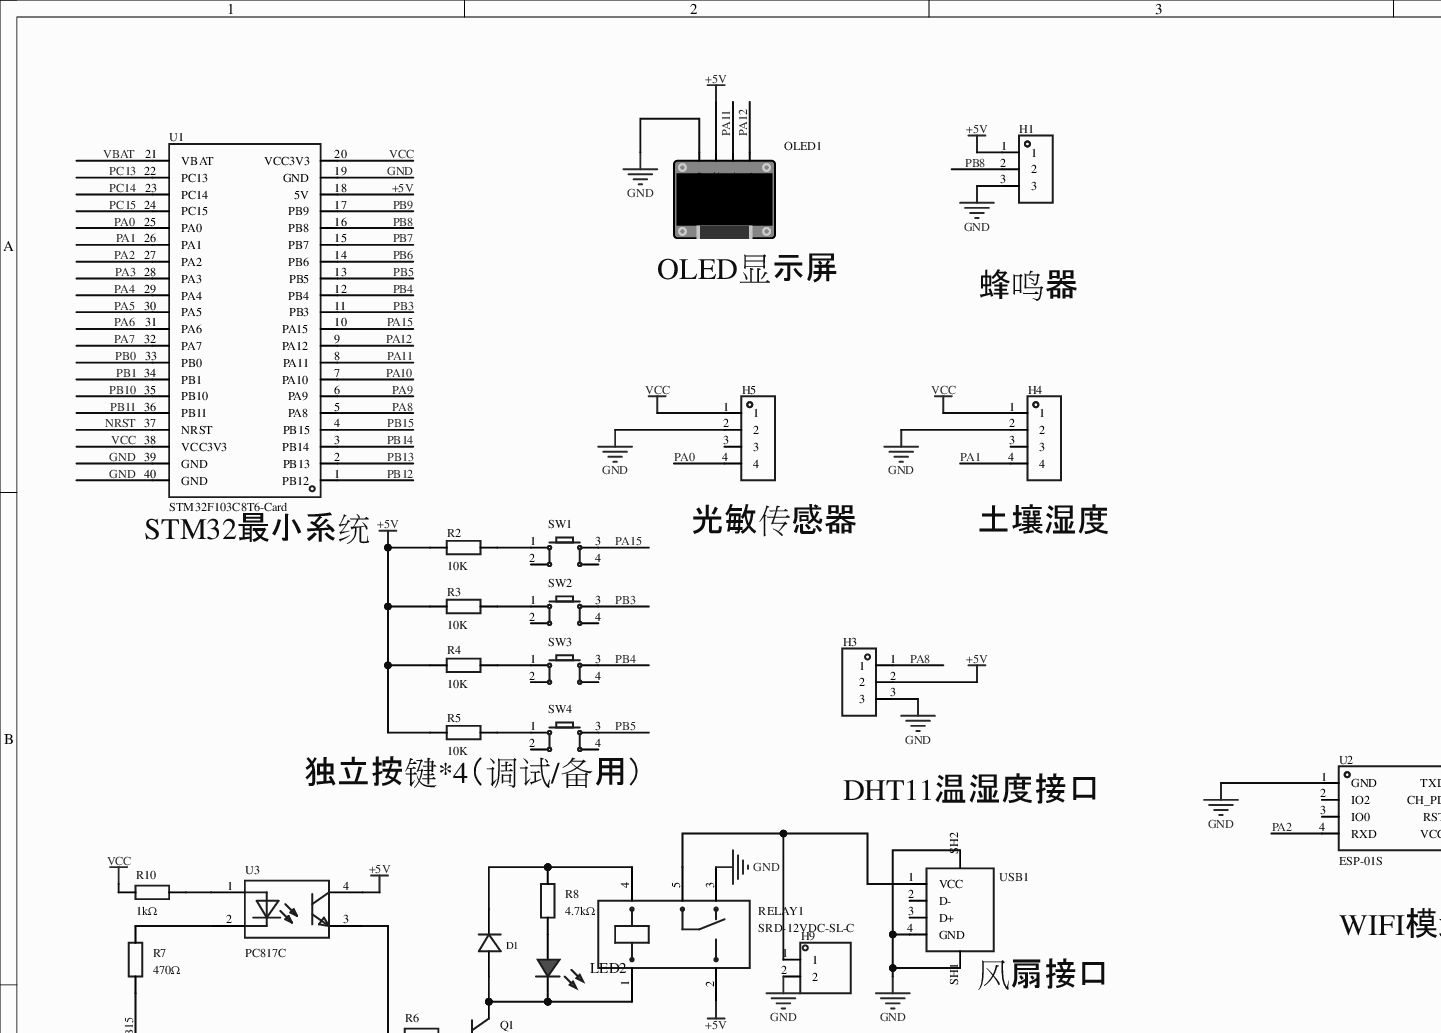
[diagram p0: MISC51241-3.schdoc, top left]
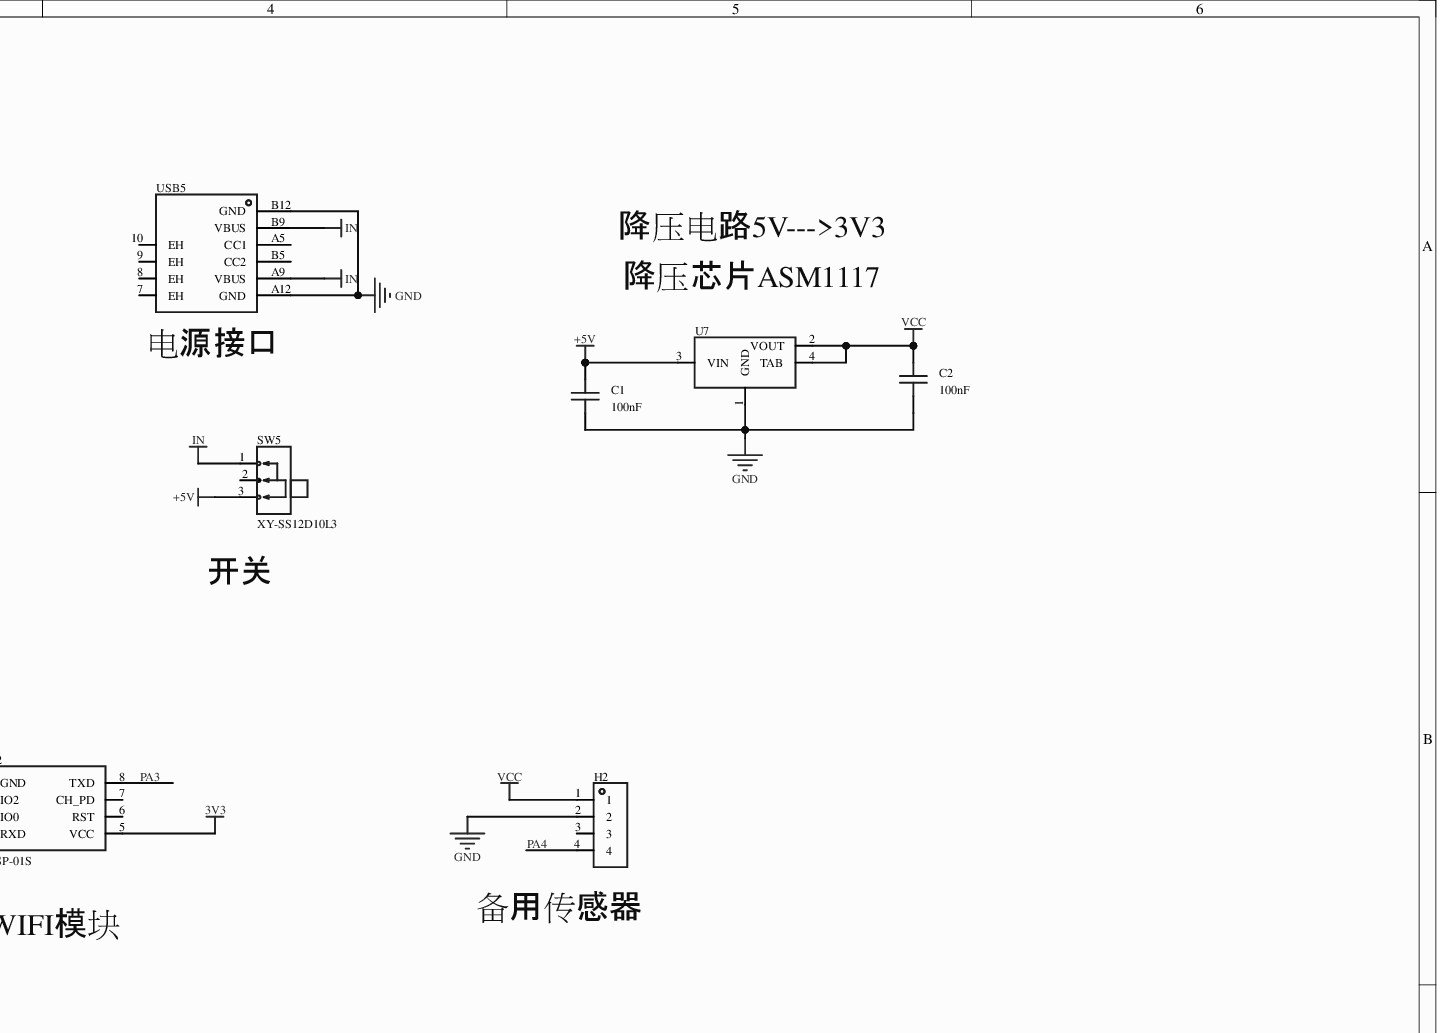
[diagram p1: MISC51241-3.schdoc, top right]
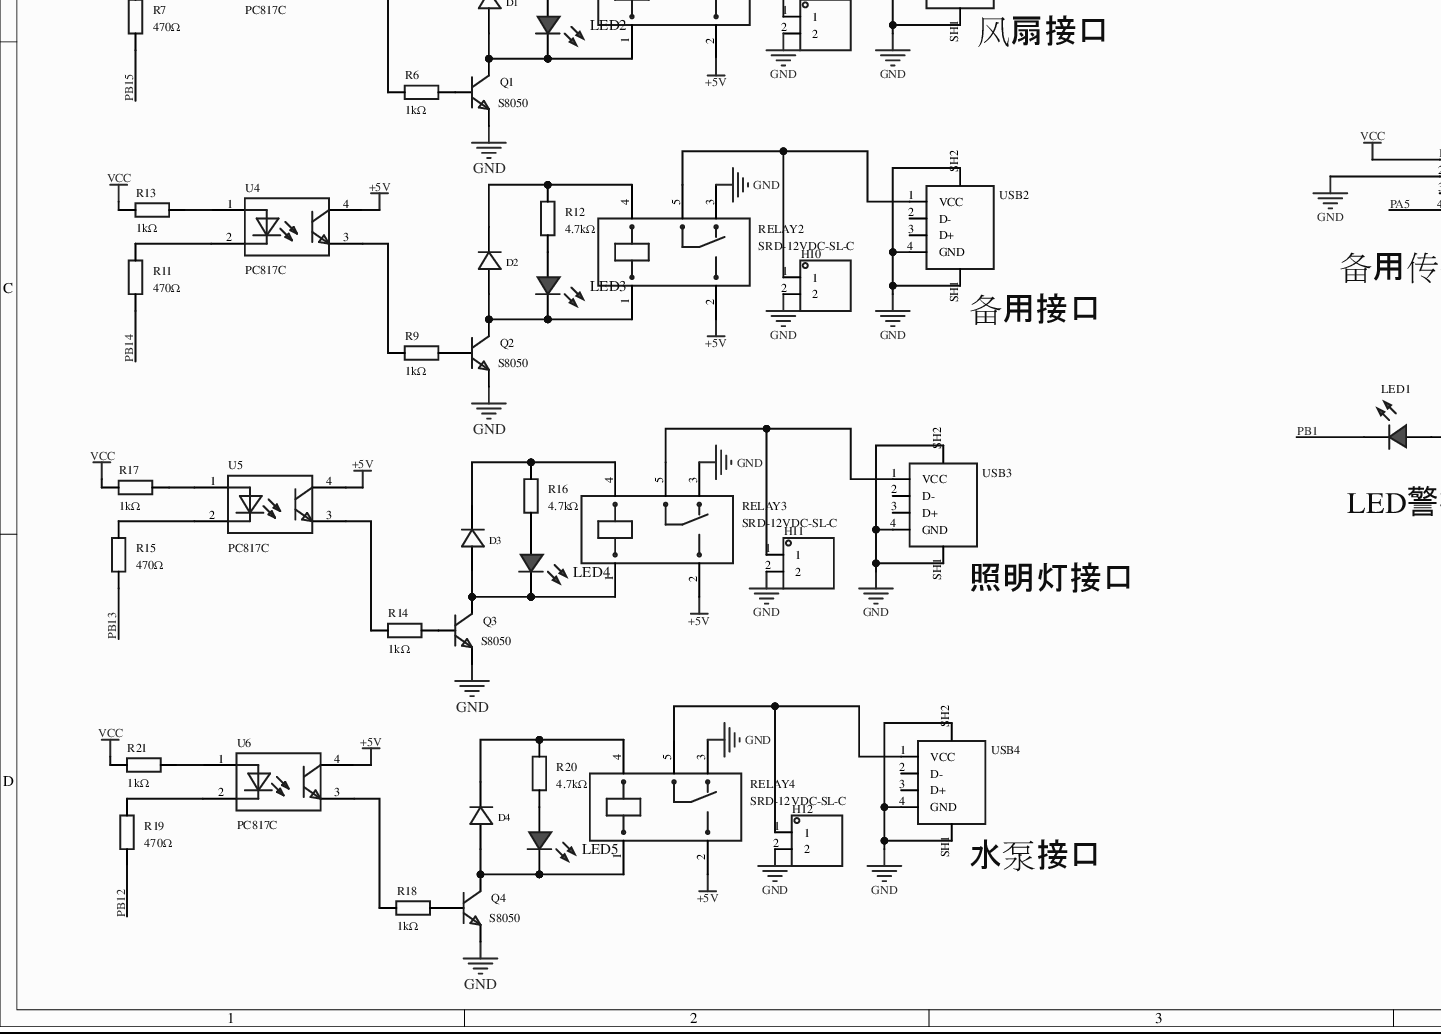
[diagram p2: MISC51241-3.schdoc, bottom left]
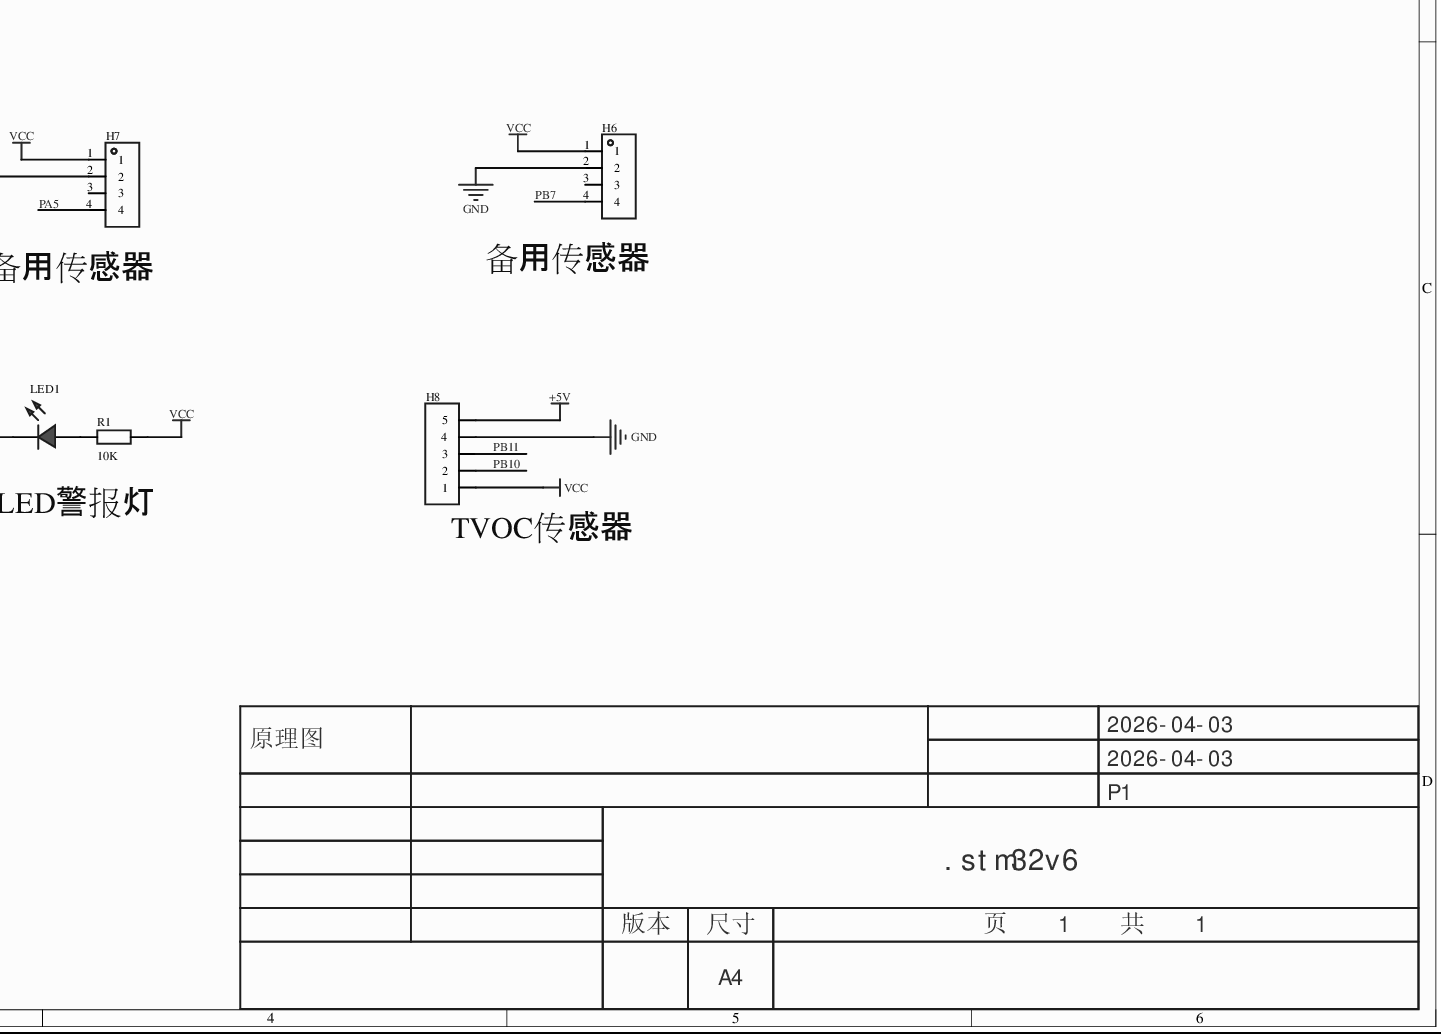
[diagram p3: MISC51241-3.schdoc, bottom right]
# Altium project MISC51241-2.PrjPcb
1 sheet, 70 parts. Net scope: global (net labels, ports and power ports of the same name join across sheets).
Board file: MISC51241.pcbdoc

## Sheet MISC51241-3.schdoc
size 420 x 297 mm; Version: V1.0; @Project Name: MISC51241; @Page Count: 1; @Update Date: 2026-04-03; @Create Date: 2026-04-03; @Schematic Name: MISC51241; @Page No: 1; @Create Time: 23:22:16; @Update Time: 17:32:40; @Board Name: MISC51241

### Parts
C1  100nF  [C0603]
C2  100nF  [C0603]
D1  US1M  [SMA_L4.4-W2.8-LS5.4-RD]  (value not drawn)
D2  US1M  [SMA_L4.4-W2.8-LS5.4-RD]  (value not drawn)
D3  US1M  [SMA_L4.4-W2.8-LS5.4-RD]  (value not drawn)
D4  US1M  [SMA_L4.4-W2.8-LS5.4-RD]  (value not drawn)
H1  (no value)  [HDR-TH_3P-P2.54-V-F]
H2  (no value)  [HDR-TH_4P-P2.54-V-F]
H3  (no value)  [HDR-TH_3P-P2.54-V-F]
H4  (no value)  [HDR-TH_4P-P2.54-V-F]
H5  (no value)  [HDR-TH_4P-P2.54-V-F]
H6  (no value)  [HDR-TH_4P-P2.54-V-F]
H7  (no value)  [HDR-TH_4P-P2.54-V-F]
H8  (no value)  [HDR-TH_5P-P2.54-V-F]
H9  (no value)  [HDR-TH_2P-P2.54-V-M-1]
H10  (no value)  [HDR-TH_2P-P2.54-V-M-1]
H11  (no value)  [HDR-TH_2P-P2.54-V-M-1]
H12  (no value)  [HDR-TH_2P-P2.54-V-M-1]
LED1  (no value)  [LED-TH_5mm]
LED2  (no value)  [LED_0603]
LED3  (no value)  [LED_0603]
LED4  (no value)  [LED_0603]
LED5  (no value)  [LED_0603]
OLED1  (no value)  [0.96OLED_4P]
Q1  S8050  [SOT-23-3_L2.9-W1.6-P1.90-LS2.8-BR]
Q2  S8050  [SOT-23-3_L2.9-W1.6-P1.90-LS2.8-BR]
Q3  S8050  [SOT-23-3_L2.9-W1.6-P1.90-LS2.8-BR]
Q4  S8050  [SOT-23-3_L2.9-W1.6-P1.90-LS2.8-BR]
R1  10K  [R0603]
R2  10K  [R0603]
R3  10K  [R0603]
R4  10K  [R0603]
R5  10K  [R0603]
R6  1kΩ  [R0603]
R7  470Ω  [R0603]
R8  4.7kΩ  [R0603]
R9  1kΩ  [R0603]
R10  1kΩ  [R0603]
R11  470Ω  [R0603]
R12  4.7kΩ  [R0603]
R13  1kΩ  [R0603]
R14  1kΩ  [R0603]
R15  470Ω  [R0603]
R16  4.7kΩ  [R0603]
R17  1kΩ  [R0603]
R18  1kΩ  [R0603]
R19  470Ω  [R0603]
R20  4.7kΩ  [R0603]
R21  1kΩ  [R0603]
RELAY1  SRD-12VDC-SL-C  [RELAY-TH_SRD-XXVDC-XL-C]
RELAY2  SRD-12VDC-SL-C  [RELAY-TH_SRD-XXVDC-XL-C]
RELAY3  SRD-12VDC-SL-C  [RELAY-TH_SRD-XXVDC-XL-C]
RELAY4  SRD-12VDC-SL-C  [RELAY-TH_SRD-XXVDC-XL-C]
SW1  (no value)  [SW-TH_4P-L6.0-W6.0-P4.50-LS6.5]
SW2  (no value)  [SW-TH_4P-L6.0-W6.0-P4.50-LS6.5]
SW3  (no value)  [SW-TH_4P-L6.0-W6.0-P4.50-LS6.5]
SW4  (no value)  [SW-TH_4P-L6.0-W6.0-P4.50-LS6.5]
SW5  XY-SS12D10L3  [SW-TH_3P-L12.7-W6.7_XY-SS12D10LXX]
U1  STM32F103C8T6-Card  [CONN-TH_L53.3-W22.9_STM32F103C8T6-CARD]
U2  ESP-01S  [WIFIM-TH_ESP-01S]
U3  PC817C  [OPTO-SMD-4_L4.6-W6.5-P2.54-LS10.3-TL]
U4  PC817C  [OPTO-SMD-4_L4.6-W6.5-P2.54-LS10.3-TL]
U5  PC817C  [OPTO-SMD-4_L4.6-W6.5-P2.54-LS10.3-TL]
U6  PC817C  [OPTO-SMD-4_L4.6-W6.5-P2.54-LS10.3-TL]
U7  (no value)  [SOT_223]
USB1  (no value)  [USB_ Type-A]
USB2  (no value)  [USB_ Type-A]
USB3  (no value)  [USB_ Type-A]
USB4  (no value)  [USB_ Type-A]
USB5  (no value)  [USB_ TYPE-C-6P]

### Nets
3V3: U2.5(VCC)
+5V: C1.2 H1.1 H3.2 H8.5 OLED1.2(VCC) R2.1 R3.1 R4.1 R5.1 RELAY1.2 RELAY2.2 RELAY3.2 RELAY4.2 SW5.3 U1.18(5V) U3.4 U4.4 U5.4 U6.4 U7.3(VIN)
GND: C1.1 C2.1 H1.3 H2.2 H3.3 H4.2 H5.2 H6.2 H7.2 H8.4 H9.2 H10.2 H11.2 H12.2 OLED1.1(GND) Q1.2 Q2.2 Q3.2 Q4.2 RELAY1.3 RELAY2.3 RELAY3.3 RELAY4.3 U1.19(GND) U1.39(GND) U1.40(GND) U2.1(GND) U7.1(GND) USB1.4(GND) USB1.SH1 USB1.SH2 USB2.4(GND) USB2.SH1 USB2.SH2 USB3.4(GND) USB3.SH1 USB3.SH2 USB4.4(GND) USB4.SH1 USB4.SH2 USB5.A12(GND) USB5.B12(GND)
IN: SW5.1 USB5.A9(VBUS) USB5.B9(VBUS)
VCC: C2.2 H2.1 H4.1 H5.1 H6.1 H7.1 H8.1 R1.2 R10.1 R13.1 R17.1 R21.1 U1.20(VCC3V3) U1.38(VCC3V3) U7.2(VOUT) U7.4(TAB)
NRST: U1.37(NRST)
PA0: H5.4 U1.25(PA0)
PA1: H4.4 U1.26(PA1)
PA2: U1.27(PA2) U2.4(RXD)
PA3: U1.28(PA3) U2.8(TXD)
PA4: H2.4 U1.29(PA4)
PA5: H7.4 U1.30(PA5)
PA6: U1.31(PA6)
PA7: U1.32(PA7)
PA8: H3.1 U1.5(PA8)
PA9: U1.6(PA9)
PA10: U1.7(PA10)
PA11: OLED1.3(SCL) U1.8(PA11)
PA12: OLED1.4(SDA) U1.9(PA12)
PA15: SW1.3 U1.10(PA15)
PB0: U1.33(PB0)
PB1: LED1.2(A) U1.34(PB1)
PB3: SW2.3 U1.11(PB3)
PB4: SW3.3 U1.12(PB4)
PB5: SW4.3 U1.13(PB5)
PB6: U1.14(PB6)
PB7: H6.4 U1.15(PB7)
PB8: H1.2 U1.16(PB8)
PB9: U1.17(PB9)
PB10: H8.2 U1.35(PB10)
PB11: H8.3 U1.36(PB11)
PB12: R19.1 U1.1(PB12)
PB13: R15.1 U1.2(PB13)
PB14: R11.1 U1.3(PB14)
PB15: R7.1 U1.4(PB15)
PC13: U1.22(PC13)
PC14: U1.23(PC14)
PC15: U1.24(PC15)
VBAT: U1.21(VBAT)
NetD1_1: D1.1(C) R8.2 RELAY1.4
NetD1_2: D1.2(A) LED2.1(C) Q1.3 RELAY1.1
NetD2_1: D2.1(C) R12.2 RELAY2.4
NetD2_2: D2.2(A) LED3.1(C) Q2.3 RELAY2.1
NetD3_1: D3.1(C) R16.2 RELAY3.4
NetD3_2: D3.2(A) LED4.1(C) Q3.3 RELAY3.1
NetD4_1: D4.1(C) R20.2 RELAY4.4
NetD4_2: D4.2(A) LED5.1(C) Q4.3 RELAY4.1
NetH9_1: H9.1 RELAY1.5 USB1.1(VCC)
NetH10_1: H10.1 RELAY2.5 USB2.1(VCC)
NetH11_1: H11.1 RELAY3.5 USB3.1(VCC)
NetH12_1: H12.1 RELAY4.5 USB4.1(VCC)
NetLED1_1: LED1.1(C) R1.1
NetLED2_2: LED2.2(A) R8.1
NetLED3_2: LED3.2(A) R12.1
NetLED4_2: LED4.2(A) R16.1
NetLED5_2: LED5.2(A) R20.1
NetQ1_1: Q1.1 R6.2
NetQ2_1: Q2.1 R9.2
NetQ3_1: Q3.1 R14.2
NetQ4_1: Q4.1 R18.2
NetR2_2: R2.2 SW1.1
NetR3_2: R3.2 SW2.1
NetR4_2: R4.2 SW3.1
NetR5_2: R5.2 SW4.1
NetR6_1: R6.1 U3.3
NetR7_2: R7.2 U3.2
NetR9_1: R9.1 U4.3
NetR10_2: R10.2 U3.1
NetR11_2: R11.2 U4.2
NetR13_2: R13.2 U4.1
NetR14_1: R14.1 U5.3
NetR15_2: R15.2 U5.2
NetR17_2: R17.2 U5.1
NetR18_1: R18.1 U6.3
NetR19_2: R19.2 U6.2
NetR21_2: R21.2 U6.1

Not connected (* = marked no-connect by the designer): H2 3; H4 3; H5 3; H6 3; H7 3; SW1 2 4; SW2 2 4; SW3 2 4; SW4 2 4; SW5 2; U2 2(IO2) 3(IO0) 6(RST) 7(CH_PD); USB1 2(D-) 3(D+); USB2 2(D-) 3(D+); USB3 2(D-) 3(D+); USB4 2(D-) 3(D+); USB5 7(EH)* 8(EH)* 9(EH)* 10(EH)* A5(CC1)* B5(CC2)*

### Notes on the sheet
- 降压电路5V--->3V3
- OLED显示屏
- 蜂鸣器
- 降压芯片ASM1117
- (near USB5) 电源接口
- (near U1) STM32最小系统
- (near H5) 光敏传感器
- (near H4) 土壤湿度
- (near SW5) 开关
- (near R5) 独立按键*4（调试/备用）
- DHT11温湿度接口
- (near USB1) 风扇接口
- WIFI模块
- (near H2) 备用传感器
- (near H7) 备用传感器
- (near H6) 备用传感器
- (near USB2) 备用接口
- LED警报灯
- (near H8) TVOC传感器
- (near USB3) 照明灯接口
- (near USB4) 水泵接口
- 2026-04-03
- 原理图
- P1
- .stm32v6
- 版本
- 尺寸
- A4
- 页    1    共    1

### Library data of the parts
C1 C2 = CAP_0603: Symbol: Capacitance; ConvertToPcb: yes; ModelId: ac125912035d415993ca9572d50418b10819f05c4eef4c71ace90d822a990e87; ModelName: C0603_L1.6-W0.8-H0.8; ModelTransform: 62.992,31.496,0,0,0,0,0,0,0; Device: CAP_0603; AddInBom: yes; Supplier Footprint: 0603; FootprintName: C0603; Value: 100nF
D1-D4 = US1M_C412437: 二极管配置:独立式;直流反向耐压(Vr):1kV;平均整流电流(Io):1A;正向压降(Vf):1.7V@1A;反向恢复时间(trr):75ns;; Manufacturer: MDD; Symbol: US1MG_C412437; 3D Model: 4f1e9ef2303f48b48aa8ce0cacf8d7b1; 3D Model Transform: 204.724,102.362,0,0,0,0,0,0,0; Diode Configuration: 独立式; Reverse Voltage (Vr): 1kV; Average Rectified Current (Io): 1A; Reverse Leakage Current: 5uA@1kV; Reverse Recovery Time (trr): 75ns; AddInBom: yes; Device: US1M_C412437; LCSC Part Name: 1kV 1A 1.7V@1A 75ns; Supplier Footprint: SMA; Datasheet: https://atta.szlcsc.com/upload/public/pdf/source/20230314/F0756B025DF5B8F55B4CA0C779F501E8.pdf; Forward Voltage (Vf@If): 1.7V@1A; Operating Temperature: -50℃~+150℃@(Tj); Supplier: LCSC; Supplier Part: C412437; Manufacturer Part: US1M; JLCPCB Part Class: Basic Part; ConvertToPcb: yes; FootprintName: SMA_L4.4-W2.8-LS5.4-RD; ModelName: SMA_L4.4-W2.8-LS5.4-RD
H1 H3 = HDR-F_2.54_1x3P: Symbol: PM254V-11-03-H85; 3D Model: f3b3cc5aae9641bf9e56fc160cef875b; 3D Model Transform: 299.9994,100,0,0,0,0,0,0,-118.11; ConvertToPcb: yes; ModelName: HDR2.54-F-LI-1X3P; Device: HDR-F_2.54_1x3P; Supplier Part: C541850; Supplier Footprint: 插件; AddInBom: yes; FootprintName: HDR-TH_3P-P2.54-V-F
H2 H5-H7 = HDR-F_2.54_1x4P: Symbol: 2.54-1*4P母; 3D Model: d187812051054f85879fcaa51a310d8e0819f05c4eef4c71ace90d822a990e87; 3D Model Transform: 419.6842,98.464,0,0,0,0,0,0,-118.11; ConvertToPcb: yes; Device: HDR-F_2.54_1x4P; Supplier Part: C2718488; Supplier Footprint: 插件; AddInBom: yes; FootprintName: HDR-TH_4P-P2.54-V-F; ModelName: HDR-TH_4P-P2.54-V-F
H4 = HDR-F_2.54_1x4P: Symbol: 2.54-1*4P母; ConvertToPcb: yes; ModelId: d187812051054f85879fcaa51a310d8e0819f05c4eef4c71ace90d822a990e87; ModelTransform: 419.6842,98.464,0,0,0,0,0,0,-118.11; Device: HDR-F_2.54_1x4P; AddInBom: yes; SupplierPart: C2718488; Supplier Footprint: 插件; FootprintName: HDR-TH_4P-P2.54-V-F; ModelName: HDR-TH_4P-P2.54-V-F
H8 = HDR-F_2.54_1x5P: Symbol: Header-Female-2.54_1x5; ConvertToPcb: yes; ModelId: f49cb6116a3d45e5a64915bf3e00773f; ModelTransform: 519.684,98.464,0,0,0,0,0,0,-124.016; Device: HDR-F_2.54_1x5P; AddInBom: yes; SupplierPart: C50950; Supplier Footprint: 插件; FootprintName: HDR-TH_5P-P2.54-V-F; ModelName: HDR-TH_5P-P2.54-V-F
H9-H12 = HDR-M_2.54_1x2P: Symbol: 210S-1*2P L=11.6MMGold-plated black; ConvertToPcb: yes; ModelId: 79b2e9f2d70a4d68a1b7098f27c6d4c50819f05c4eef4c71ace90d822a990e87; ModelName: HDR-M-2.54_1x2; ModelTransform: 200,100,0,0,0,0,0,0,-118.11; Device: HDR-M_2.54_1x2P; AddInBom: yes; SupplierPart: C124375; Supplier Footprint: 插件; FootprintName: HDR-TH_2P-P2.54-V-M-1
LED1 = LED_TH-R_5mm: ConvertToPcb: yes; ModelId: fe9cea1bdf7642cd8d9a5077ed0e2b580819f05c4eef4c71ace90d822a990e87; ModelName: LED-TH_BD5.9-P2.54-RD_RED; ModelTransform: 222.16,238.98,581.81,180,0,0,-6,0,-220; Symbol: LED_TH-R; Device: LED_TH-R_5mm; AddInBom: yes; FootprintName: LED-TH_5mm; Supplier Footprint: 插件
LED2-LED5 = LED_0603-R: Symbol: LED_R; Convert to PCB: yes; 3D Model: dd8257b0d61a4cd7b68939a056e08095; 3D Model Transform: 58.72,29.4,22.03,0,0,0,0,0,0; ModelName: LED-0603_R; Device: LED_0603-R; Add into BOM: yes; Supplier Footprint: 0603; FootprintName: LED_0603
OLED1 = 0.96OLED模块_4P: ConvertToPcb: yes; ModelId: 79c000fdb68d45a296c2e9bedf4f9055; ModelTransform: 1393.69792,1318.895,0,0,0,0,0,-560.079,-137.795; Symbol: 0.96OLED模块_4P; Device: 0.96OLED模块_4P; AddInBom: yes; FootprintName: 0.96OLED_4P; Supplier Footprint: 插件; ModelName: 0.96OLED_4P
Q1-Q4 = S8050_C105433: 晶体管类型:NPN;集射极击穿电压(Vceo):25V;集电极电流(Ic):500mA;功率(Pd):300mW;直流电流增益(hFE@Ic,Vce):120@50mA,1V;; Manufacturer: CJ(江苏长电/长晶); 3D Model: 89cb27a44ab2466697082bb9fd73a7d0; 3D Model Transform: 110.236,114.173,0,180,0,0,-0.005,0.0005,0; Transistor Type: NPN; Collector-Emitter Breakdown Voltage (Vceo): 25V; Collector Current (Ic): 500mA; Power Dissipation (Pd): 300mW; Collector Cut-Off Current (Icbo): 100nA; Collector-Emitter Saturation Voltage (VCE(sat)@Ic,Ib): 600mV@500mA,50mA; Transition Frequency (fT): 150MHz; AddInBom: yes; ModelName: SOT-23-3L_L2.9-W1.6-H1.1-LS2.8-P0.95; Symbol: S8050_C105433; Device: S8050_C105433; LCSC Part Name: NPN 25V 500mA L档 120-200; Supplier Part: C105433; Manufacturer Part: S8050; Supplier Footprint: SOT-23; JLCPCB Part Class: Extended Part; Datasheet: https://atta.szlcsc.com/upload/public/pdf/source/20170415/1492237762328.pdf; Supplier: LCSC; DC Current Gain (hFE@Ic,Vce): 120@50mA,1V; Operating Temperature: +150℃@(Tj); ConvertToPcb: yes; FootprintName: SOT-23-3_L2.9-W1.6-P1.90-LS2.8-BR
R1-R5 R8 R12 R16 R20 = Res_0603: Symbol: 电阻; 3D Model: fc143cca1e79419f9cd78b61e9279f080819f05c4eef4c71ace90d822a990e87; 3D Model Transform: 31.8897,63.7794,0,90,0,0,0,0,0; ConvertToPcb: yes; Device: Res_0603; Supplier Footprint: 0603; AddInBom: yes; FootprintName: R0603; ModelName: R0603
  R1-R5: Value: 10K
  R8 R12 R16 R20: Value: 4.7kΩ
R6 R7 R9-R11 R13-R15 R17-R19 R21 = 0603WAF1001T5E: 电阻类型:厚膜电阻;阻值:1kΩ;精度:±1%;功率:100mW;; Manufacturer: UNI-ROYAL(厚声); 3D Model: fc143cca1e79419f9cd78b61e9279f08; 3D Model Transform: 31.8897,63.7794,0,90,0,0,0,0,0; Tolerance: ±1%; Power(Watts): 100mW; Temperature Coefficient: ±100ppm/℃; Overload Voltage (Max): 75V; AddInBom: yes; Symbol: 0603WAF1001T5E; Device: 0603WAF1001T5E; LCSC Part Name: 1kΩ ±1% 100mW; Manufacturer Part: 0603WAF1001T5E; Supplier Footprint: 0603; JLCPCB Part Class: Basic Part; Datasheet: https://atta.szlcsc.com/upload/public/pdf/source/20200306/C422600_1E6D84923E4A46A82E41ADD87F860B5C.pdf; Supplier: LCSC; Type: 厚膜电阻; Operating Temperature Range: -55℃~+155℃; ConvertToPcb: yes; FootprintName: R0603; ModelName: R0603
  R6 R9 R10 R13 R14 R17 R18 R21: Supplier Part: C21190; Value: 1kΩ
  R7 R11 R15 R19: Value: 470Ω
RELAY1-RELAY4 = SRD-12VDC-SL-C: 线圈电压:12V;引脚数:5;触点形式:一组转换:1C(单刀双掷-转换);触点容量(电阻负载):-;; Manufacturer: 松乐; 3D Model: d0eda9b8bf8746d18ae810ab88dc78e7; 3D Model Transform: 755.904,614.172,0,0,0,0,34.882,0,-137.795; Coil Voltage: 12V; Coil Type: 非极化-单线圈; Pin Number: 5; Maximum Switching Current: 15A; Maximum Switching Voltage: 250V@AC; Coil Rated Power: 360mW; Coil Resistance: 400Ω; Operate Time: 10ms; Contact Resistance: 100mΩ; AddInBom: yes; ModelName: RELAY-TH_L19.2-W15.6-H15.8; Symbol: SRD-12VDC-SL-C; Device: SRD-12VDC-SL-C; LCSC Part Name: 12V继电器 单刀双掷 蓝色; Supplier Part: C30431; Manufacturer Part: SRD-12VDC-SL-C; Supplier Footprint: 插件,15.6x19.2mm; JLCPCB Part Class: Extended Part; Datasheet: https://atta.szlcsc.com/upload/public/pdf/source/20180525/C30431_534ADD4B54993D382CD0EDFAB06D3E7F.pdf; Supplier: LCSC; Contact Form: 一组转换:1C(单刀双掷-转换); Contact Rating: -; Release Time: 10ms; ConvertToPcb: yes; FootprintName: RELAY-TH_SRD-XXVDC-XL-C
SW1-SW4 = Key_TH_6x6x6: 触点电流:50mA;额定电压(DC):12V;绝缘电阻:100MΩ;电路结构:单刀单掷;安装方式:直插;按钮形状:圆形按钮;按钮/盖帽颜色:黑色;作用力:260gf@±30gf;工作温度:-25℃~+70℃;引脚样式:PC引脚;开关长度:6mm;开关宽度:6mm;开关高度:6mm;带支架:否;; Symbol: 轻触按键; AddInBom: yes; ModelId: 20eee248bc684ccd8cbdbb1d0d91ec6f0819f05c4eef4c71ace90d822a990e87; ModelName: SW-TH_4P-L6.0-W6.0-H5.0-LS6.5-P4.50; ModelTransform: 236.22,323.03,0,90,0,0,0,0,-137.795; Device: Key_TH_6x6x6; ConvertToPcb: yes; FootprintName: SW-TH_4P-L6.0-W6.0-P4.50-LS6.5; Supplier Footprint: 插件
SW5 = XY-SS12D10L3: 拨动开关,立式直脚两档,插件,单排正拨,柄长3mm; Manufacturer: XYECONN(辛译); AddInBom: yes; Symbol: XY-SS12D10L3; Device: XY-SS12D10L3; LCSC Part Name: 拨动开关,立式直脚两档,插件,单排正拨,柄长3mm; SupplierPart: C49652929; ManufacturerPart: XY-SS12D10L3; Supplier Footprint: 插件; JLCPCB Part Class: Extended Part; Datasheet: https://item.szlcsc.com/datasheet/XY-SS12D10L3/52215304.html; Supplier: LCSC; ConvertToPcb: yes; FootprintName: SW-TH_3P-L12.7-W6.7_XY-SS12D10LXX
U1 = STM32F103C8T6-Card: AddInBom: yes; Symbol: STM32F103C8T6-CARD; Device: STM32F103C8T6-Card; LCSC Part Name: STM32F103C8T6-Card; SupplierPart: C9900077949; ManufacturerPart: STM32F103C8T6-Card; Supplier Footprint: 插件; Supplier: LCSC; ConvertToPcb: yes; FootprintName: CONN-TH_L53.3-W22.9_STM32F103C8T6-CARD
U2 = ESP-01S_C111009: 3D Model: eb7175da78ae48b3b1568cfe3027405f0819f05c4eef4c71ace90d822a990e87; 3D Model Transform: 582.676,976.37608,0,0,0,0,0,388.346,-118.11; AddInBom: yes; Symbol: ESP-01S; Device: ESP-01S_C111009; LCSC Part Name: ESP-01S; Supplier Part: C111009; Manufacturer Part: ESP-01S; Supplier Footprint: -; JLCPCB Part Class: Extended Part; Supplier: LCSC; ConvertToPcb: yes; FootprintName: WIFIM-TH_ESP-01S; ModelName: WIFIM-TH_ESP-01S
U3-U6 = PC817C_C3025164: Manufacturer: GOODWORK(固得沃克); 3D Model: 2d94a81bf94f4608bff03a785b63c361; 3D Model Transform: 401.574,181.102,0,0,0,0,0,0,0; AddInBom: yes; ModelName: OPTO-SMD-4_L4.6-W6.5-H3.6-LS10.2-P2.54; Symbol: PC817C_C3025164; Device: PC817C_C3025164; LCSC Part Name: C档; Supplier Part: C3025164; Manufacturer Part: PC817C; Supplier Footprint: SMD-4P; JLCPCB Part Class: Extended Part; Datasheet: https://atta.szlcsc.com/upload/public/pdf/source/20220530/3FD5D572B823BA05C967330A07ECF74F.pdf; Supplier: LCSC; ConvertToPcb: yes; FootprintName: OPTO-SMD-4_L4.6-W6.5-P2.54-LS10.3-TL
U7 = AMS1117: Symbol: AMS1117_OLD; AddInBom: yes; ModelId: 925194bf9823436183a3e0b978a8d0760819f05c4eef4c71ace90d822a990e87; ModelName: SOT-223-4P_L6.5-W3.5-H1.6-LS7.0-P2.30; ModelTransform: 279.84,255.85,68.86,90,0,0,0,0,0; Device: AMS1117; ConvertToPcb: yes; FootprintName: SOT_223
USB1-USB4 = USB_ Type-A: AddInBom: yes; ModelId: 0a0bfc60af8549fa93b7465d8aaf02b10819f05c4eef4c71ace90d822a990e87; ModelName: USB-A-TH__USB-AF-90; ModelTransform: 612.05,551.18,446.85,0,0,0,0,-15.75,-157.48; Symbol: USB_Type-A; Device: USB_ Type-A; ConvertToPcb: yes; FootprintName: USB_ Type-A; Supplier Footprint: 插件
USB5 = USB_ Type-C-6P: AddInBom: yes; ModelId: d4f492a4e6024845a13b3f6a4ef2d2cb0819f05c4eef4c71ace90d822a990e87; ModelName: USB-SMD_U262-061N-4BVC11; ModelTransform: 352.362,281.496,0,0,0,0,0,-47.244,-39.37; Symbol: USB_ TYPE-C-6P; Device: USB_ Type-C-6P; Supplier Footprint: SMD; ConvertToPcb: yes; FootprintName: USB_ TYPE-C-6P